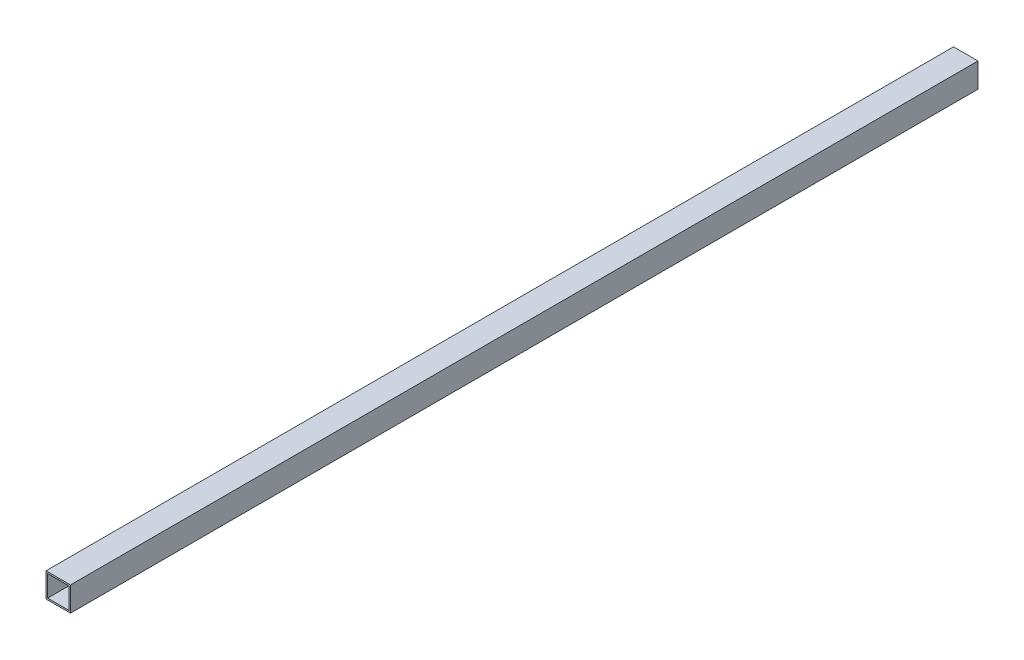
SolidWorks part; units mm, degrees
ref_plane "前视基准面" through (0, 0, 0) normal (0, 0, 1) x (1, 0, 0)
ref_plane "上视基准面" through (0, 0, 0) normal (0, 1, 0) x (1, 0, 0)
ref_plane "右视基准面" through (0, 0, 0) normal (1, 0, 0) x (0, 0, -1)
sketch "草图1" plane through (0, 0, 0) normal (0, 0, 1) x (1, 0, 0)
  line L0 (13, 13) -> (-13, 13)
  line L1 (15, -15) -> (-15, -15)
  line L2 (15, -15) -> (15, 15)
  line L3 (15, 15) -> (-15, 15)
  line L4 (-15, -15) -> (-15, 15)
  line L5 (15, -15) -> (-15, 15) construction
  line L6 (15, 15) -> (-15, -15) construction
  line L7 (-13, -13) -> (-13, 13)
  line L8 (13, -13) -> (-13, -13)
  line L9 (13, -13) -> (13, 13)
  point P0 (0, 0)
  dimension "D1" = 30
  dimension "D2" = 2
extrude "凸台-拉伸1" add sketch "草图1" along normal mid plane 1112
